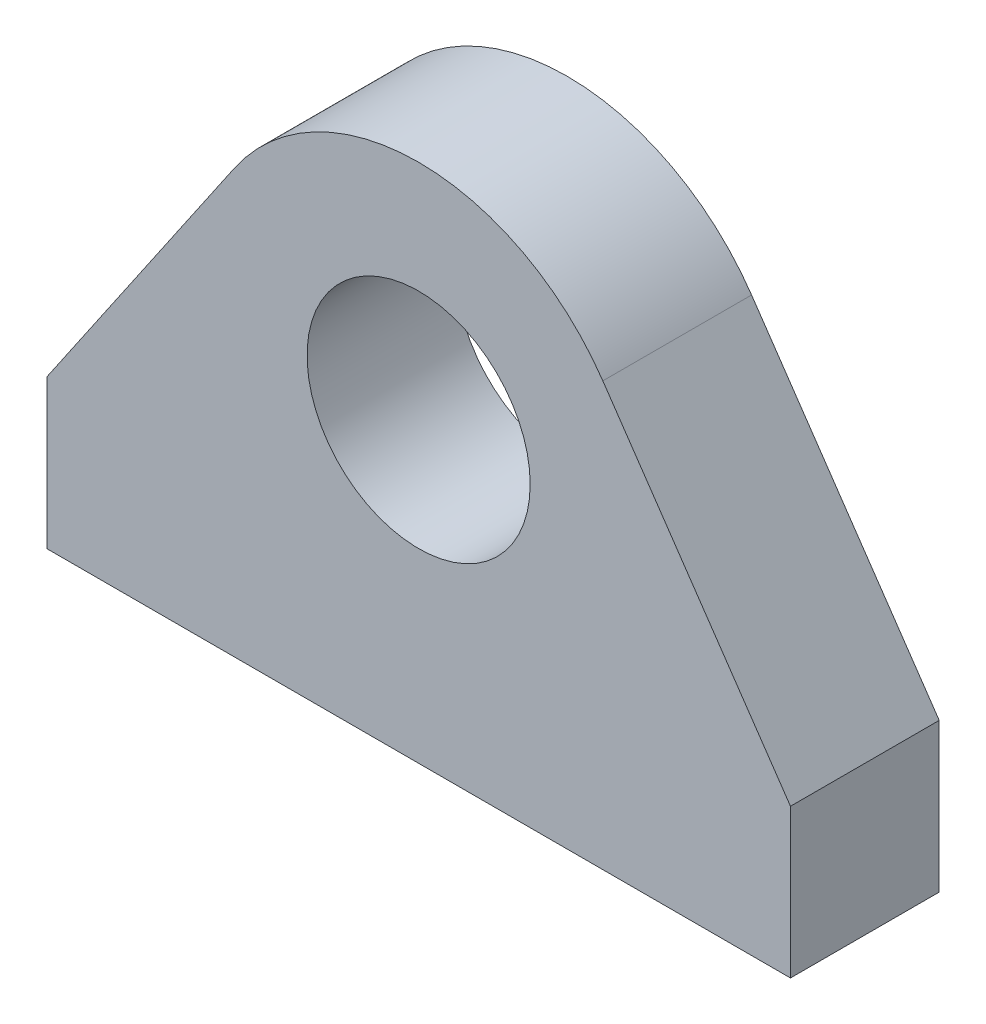
from build123d import *

# Parameters (mm, degrees)
SKETCH_1_R      = 7.5
EXTRUDE_1_DEPTH = 10


with BuildPart() as part:
    # 草图1 → 凸台-拉伸1 (new body)
    with BuildSketch(Plane.XY):
        with BuildLine():
            Line((25, -20), (-25, -20))
            Line((-25, -20), (-25, -10))
            Line((-25, -10), (-12.384968229, 8.462420573))
            ThreePointArc((-12.384968229, 8.462420573), (0, 15), (12.384968229, 8.462420573))
            Line((12.384968229, 8.462420573), (25, -10))
            Line((25, -10), (25, -20))
        make_face()
        Circle(SKETCH_1_R, mode=Mode.SUBTRACT)
    extrude(amount=EXTRUDE_1_DEPTH)


solid = part.part
